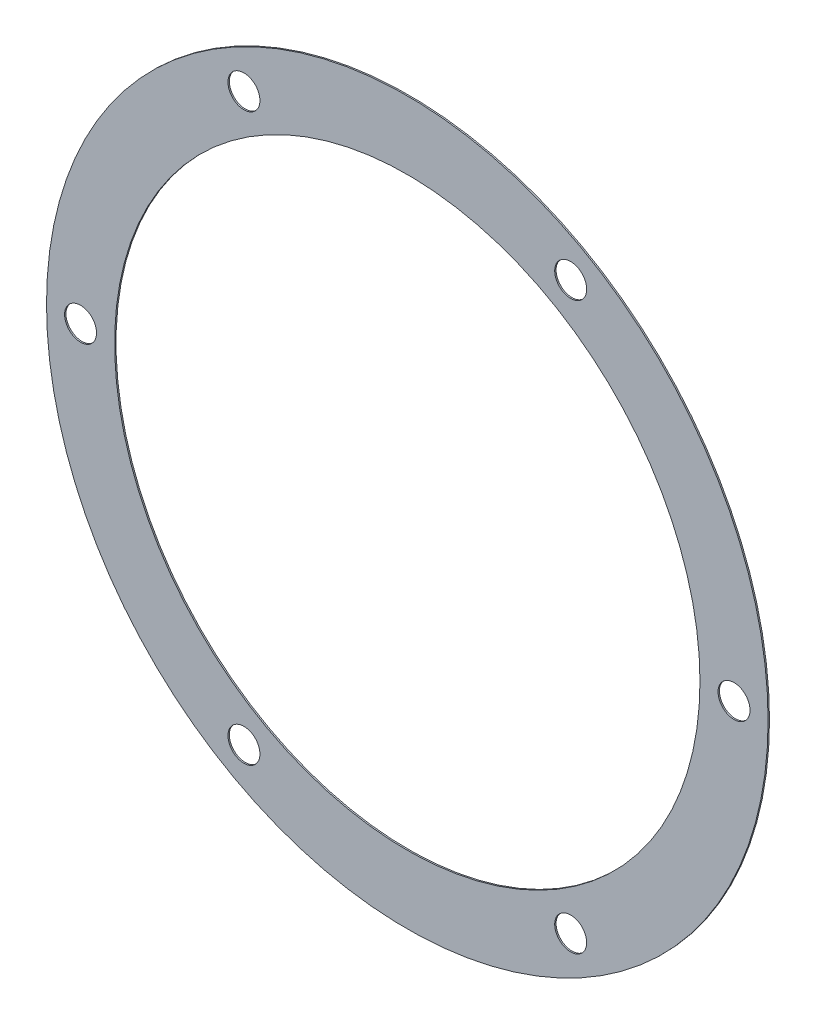
from build123d import *

# Parameters (mm, degrees)
SKETCH1_R           = 259.5
SKETCH1_R_2         = 210.5
BOSS_EXTRUDE1_DEPTH = 1
CUT_EXTRUDE1_REACH  = 368.99
SKETCH2_R           = 11.5
CIRPATTERN1_COUNT   = 6


with BuildPart() as part:
    # Sketch1 → Boss-Extrude1 (new body)
    with BuildSketch(Plane.XY):
        Circle(SKETCH1_R)
        Circle(SKETCH1_R_2, mode=Mode.SUBTRACT)
    extrude(amount=BOSS_EXTRUDE1_DEPTH)

    # Sketch2 → Cut-Extrude1 (cut, up to next)
    with BuildSketch(Plane.XY.offset(1), mode=Mode.PRIVATE) as cut_extrude1_sk1:
        with Locations((-235, 0)):
            Circle(SKETCH2_R)
    cut_extrude1_tool1 = extrude(cut_extrude1_sk1.sketch, amount=-CUT_EXTRUDE1_REACH, mode=Mode.PRIVATE) & part.part
    cut_extrude1 = cut_extrude1_tool1.solids().sort_by_distance((-235, 0, 1))[0]
    add(cut_extrude1, mode=Mode.SUBTRACT)

    # CirPattern1: Cut-Extrude1 ×6 about axis
    cirpattern1_axis = Axis((0, 0, 0), (0, 0, 1))
    for i in range(1, CIRPATTERN1_COUNT):
        add(cut_extrude1.rotate(cirpattern1_axis, i * 360 / CIRPATTERN1_COUNT), mode=Mode.SUBTRACT)


solid = part.part
